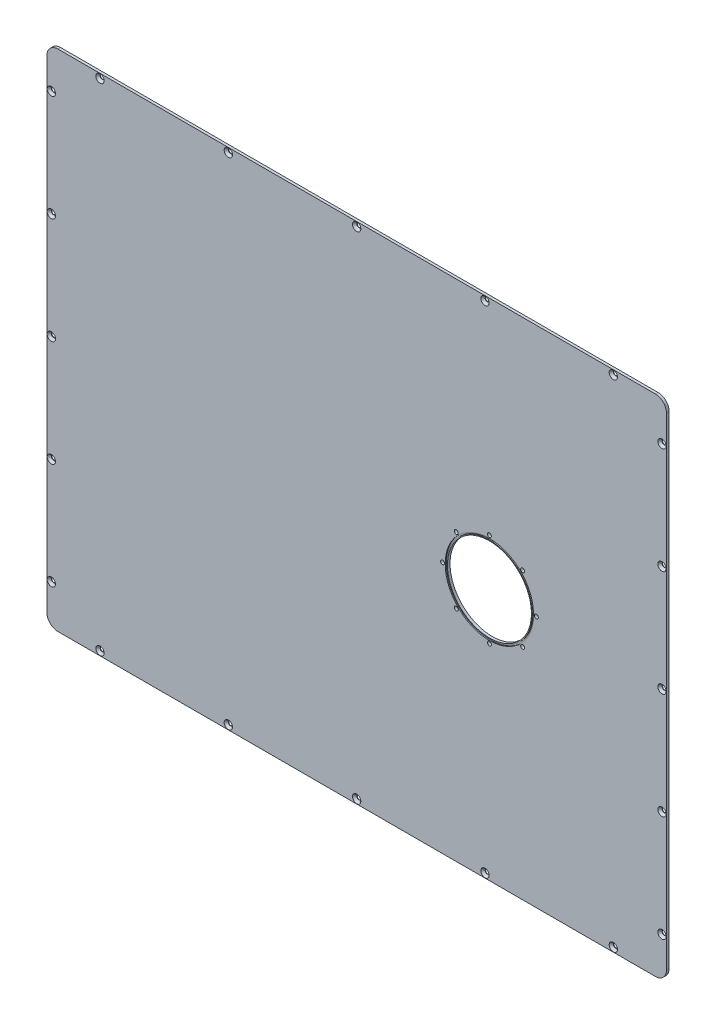
SolidWorks part; units mm, degrees
ref_plane "前视基准面" through (0, 0, 0) normal (0, 0, 1) x (1, 0, 0)
ref_plane "上视基准面" through (0, 0, 0) normal (0, 1, 0) x (1, 0, 0)
ref_plane "右视基准面" through (0, 0, 0) normal (1, 0, 0) x (0, 0, -1)
sketch "草图1" plane through (0, 0, 0) normal (0, 0, 1) x (1, 0, 0)
  line L8 (227.0123, 39.0187) -> (227.0123, 584.0187)
  line L9 (214.5123, 596.5187) -> (-460.4877, 596.5187)
  line L10 (-472.9877, 584.0187) -> (-472.9877, 39.0187)
  line L11 (-460.4877, 26.5187) -> (214.5123, 26.5187)
  arc A8 (214.5123, 26.5187) -> (227.0123, 39.0187) centre (214.5123, 39.0187) ccw
  arc A9 (227.0123, 584.0187) -> (214.5123, 596.5187) centre (214.5123, 584.0187) ccw
  arc A10 (-460.4877, 596.5187) -> (-472.9877, 584.0187) centre (-460.4877, 584.0187) ccw
  arc A11 (-472.9877, 39.0187) -> (-460.4877, 26.5187) centre (-460.4877, 39.0187) ccw
extrude "凸台-拉伸1" add sketch "草图1" along normal blind 3
hole_wizard "M4 锥坑平头螺钉的锥形沉头孔1" positions "草图2" profile "草图3" countersink size "M4" standard "ISO"
sketch "草图2" plane through (0, 0, 3) normal (0, 0, 1) x (1, 0, 0)
  point P0 (222.0123, 71.5187)
  point P3 (222.0123, 191.5187)
  point P6 (222.0123, 311.5187)
  point P9 (222.0123, 431.5187)
  point P12 (222.0123, 551.5187)
  point P15 (167.0123, 591.5187)
  point P18 (22.0123, 591.5187)
  point P21 (-122.9877, 591.5187)
  point P24 (-267.9877, 591.5187)
  point P27 (-412.9877, 591.5187)
  point P30 (-467.9877, 551.5187)
  point P33 (-467.9877, 431.5187)
  point P36 (-467.9877, 311.5187)
  point P39 (-467.9877, 191.5187)
  point P42 (-467.9877, 71.5187)
  point P45 (-412.9877, 31.5187)
  point P48 (-267.9877, 31.5187)
  point P51 (-122.9877, 31.5187)
  point P54 (22.0123, 31.5187)
  point P57 (167.0123, 31.5187)
sketch "草图3" plane through (222.0123, 71.5187, 3) normal (1, 0, 0) x (0, -1, 0)
  line L0 (0, 0) -> (0, 11.4519)
  line L1 (0, 11.4519) -> (2.25, 10.1)
  line L2 (2.25, 10.1) -> (2.25, 2.45)
  line L3 (2.25, 2.45) -> (4.7, 0)
  line L5 (4.7, 0) -> (0, 0)
  line L6 (-2.25, 2.45) -> (-4.7, 0) construction
  line L10 (0, 11.4519) -> (-2.25, 10.1) construction
  line L11 (0, -6.35) -> (0, 107.95) construction
  dimension "孔直径" = 4.5
  dimension "孔深度" = 10.1
  dimension "近端锥形沉头孔直径" = 9.4
  dimension "近端锥形沉头孔角度" = 90
  dimension "导头角度" = 118
sketch "草图4" plane through (0, 0, 3) normal (0, 0, 1) x (1, 0, 0)
  circle A0 centre (27.0123, 311.5187) radius 47.5
  dimension "D1" = 95
extrude "切除-拉伸1" cut sketch "草图4" against normal blind 12
sketch "草图5" plane through (0, 0, 3) normal (0, 0, 1) x (1, 0, 0)
  circle A0 centre (27.0123, 311.5187) radius 50
  circle A1 centre (27.0123, 311.5187) radius 48.5
  dimension "D1" = 97
  dimension "D2" = 100
extrude "切除-拉伸2" cut sketch "草图5" against normal blind 1.2
sketch "草图6" plane through (0, 0, 3) normal (0, 0, 1) x (1, 0, 0)
  circle A0 centre (27.0123, 258.5187) radius 2.25
  circle A1 centre (-10.4643, 274.042) radius 2.25
  circle A2 centre (-25.9877, 311.5187) radius 2.25
  circle A3 centre (-10.4643, 348.9954) radius 2.25
  circle A4 centre (27.0123, 364.5187) radius 2.25
  circle A5 centre (64.489, 348.9954) radius 2.25
  circle A6 centre (80.0123, 311.5187) radius 2.25
  circle A7 centre (64.489, 274.042) radius 2.25
  dimension "D1" = 4.5
extrude "切除-拉伸3" cut sketch "草图6" against normal blind 10
